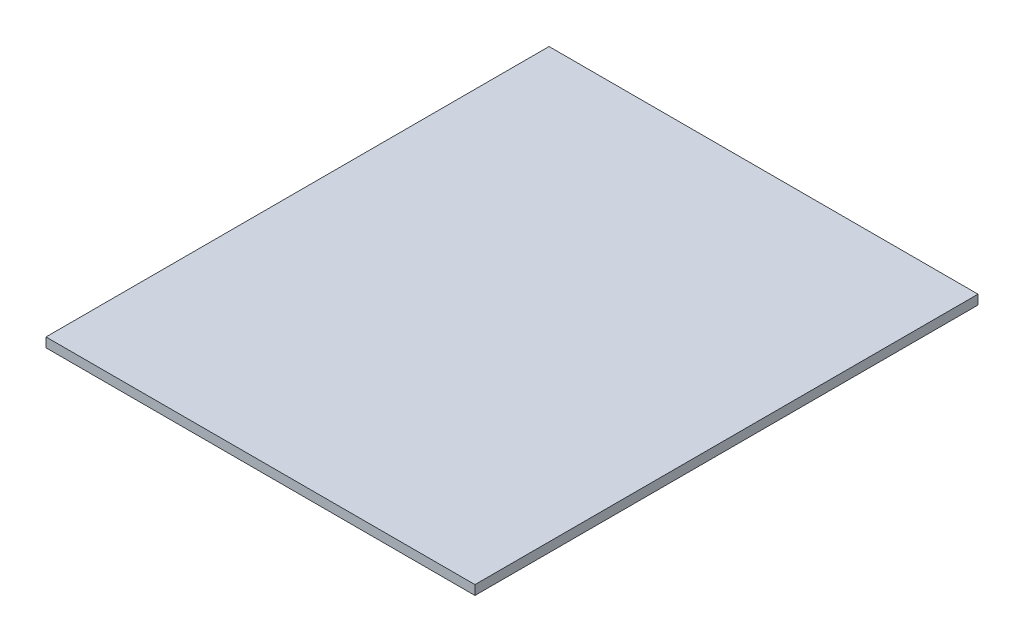
from build123d import *

# Parameters (mm, degrees)
SKETCH1_W           = 463.2
SKETCH1_H           = 543.2
BOSS_EXTRUDE1_DEPTH = 10.2


with BuildPart() as part:
    # Sketch1 → Boss-Extrude1 (new body)
    with BuildSketch(Plane(origin=(0, 0, 0), x_dir=(1, 0, 0), z_dir=(0, 1, 0))):
        with Locations((231.6, 271.6)):
            Rectangle(SKETCH1_W, SKETCH1_H)
    extrude(amount=BOSS_EXTRUDE1_DEPTH)


solid = part.part
